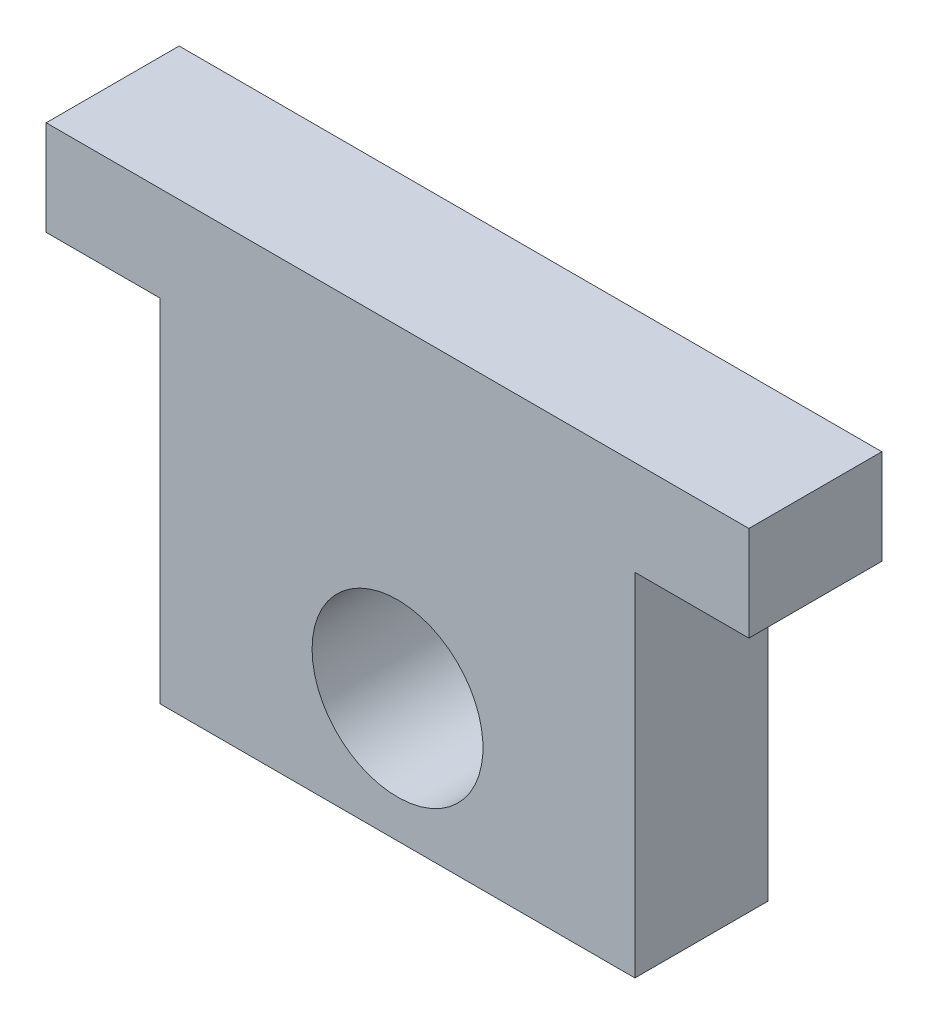
SolidWorks part; units mm, degrees
ref_plane "前视基准面" through (0, 0, 0) normal (0, 0, 1) x (1, 0, 0)
ref_plane "上视基准面" through (0, 0, 0) normal (0, 1, 0) x (1, 0, 0)
ref_plane "右视基准面" through (0, 0, 0) normal (1, 0, 0) x (0, 0, -1)
sketch "草图1" plane through (0, 0, 0) normal (0, 0, 1) x (1, 0, 0)
  line L1 (-25, -23.5) -> (25, -23.5)
  line L2 (-25, -23.5) -> (-25, 23.5)
  line L3 (-25, 23.5) -> (25, 23.5)
  line L4 (25, -23.5) -> (25, 23.5)
  line L5 (-25, -23.5) -> (25, 23.5) construction
  line L6 (-25, 23.5) -> (25, -23.5) construction
  point P0 (0, 0)
  dimension "D1" = 50
  dimension "D2" = 47
extrude "凸台-拉伸1" add sketch "草图1" along normal mid plane 14
sketch "草图2" plane through (0, 0, -7) normal (0, 0, -1) x (-1, 0, 0)
  line L0 (25, -23.5) -> (-25, -23.5) construction
  circle A0 centre (0, -10.5) radius 9
  dimension "D1" = 18
  dimension "D2" = 13
extrude "切除-拉伸1" cut sketch "草图2" against normal up to next
sketch "草图4" plane through (0, 23.5, 0) normal (0, 1, 0) x (1, 0, 0)
  line L0 (25, -7) -> (-25, -7) construction
  line L1 (25, 7) -> (37, 7)
  line L2 (25, 7) -> (25, -7)
  line L3 (25, -7) -> (37, -7)
  line L4 (37, 7) -> (37, -7)
  line L5 (-25, 7) -> (-37, 7)
  line L6 (-25, 7) -> (-25, -7)
  line L7 (-25, -7) -> (-37, -7)
  line L8 (-37, 7) -> (-37, -7)
  dimension "D1" = 12
extrude "凸台-拉伸2" add sketch "草图4" against normal blind 10
